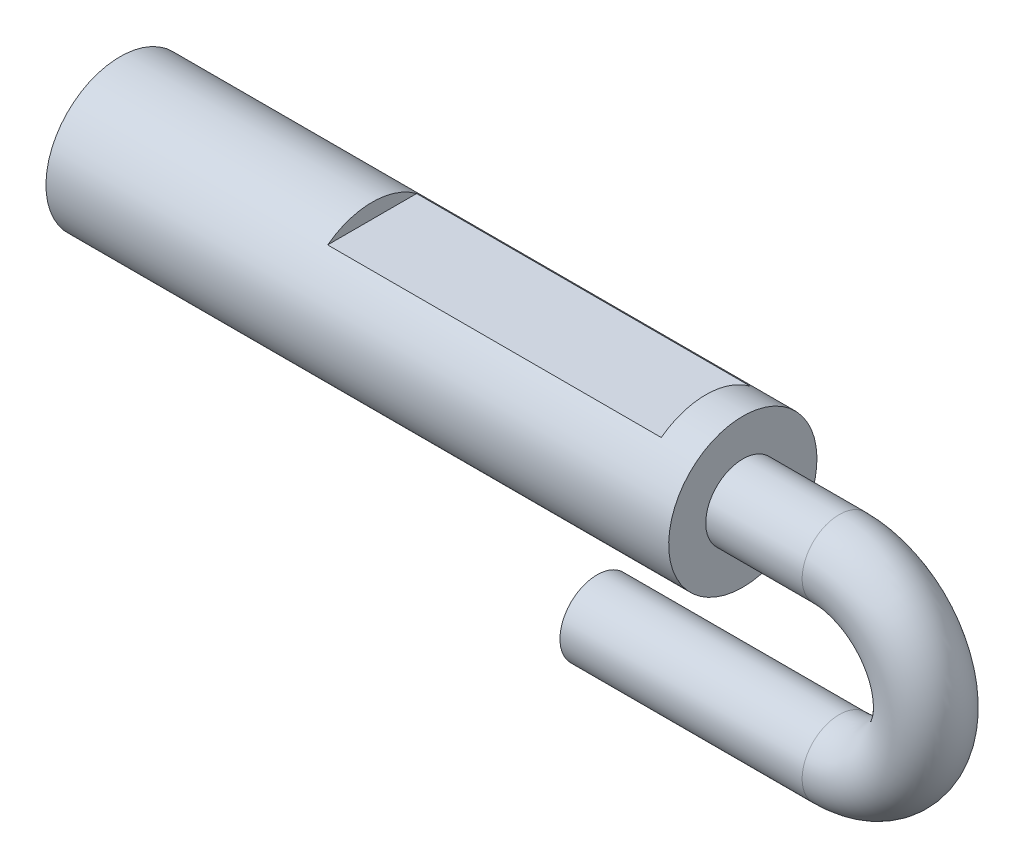
SolidWorks part; units mm, degrees
material "45"
ref_plane "前视基准面" through (0, 0, 0) normal (0, 0, 1) x (1, 0, 0)
ref_plane "上视基准面" through (0, 0, 0) normal (0, 1, 0) x (1, 0, 0)
ref_plane "右视基准面" through (0, 0, 0) normal (1, 0, 0) x (0, 0, -1)
sketch "草图1" plane through (0, 0, 0) normal (0, 0, 1) x (1, 0, 0)
  line L1 (-42, 0) -> (42, 0)
  line L2 (-42, 0) -> (-42, 10)
  line L3 (-42, 10) -> (42, 10)
  line L4 (42, 0) -> (42, 10)
  point P4 (0, 0)
  dimension "D1" = 10
  dimension "D2" = 84
revolve "旋转1" add sketch "草图1" angle 360 about L1
ref_plane "基准面1" through (0, 10, 0) normal (0, 1, 0) x (1, 0, 0)
sketch "草图2" plane through (0, 10, 0) normal (0, 1, 0) x (1, 0, 0)
  line L0 (42, -10) -> (42, 10) construction
  line L1 (-8, 17.2018) -> (37, 17.2018)
  line L2 (-8, 17.2018) -> (-8, -23.2445)
  line L3 (-8, -23.2445) -> (37, -23.2445)
  line L4 (37, 17.2018) -> (37, -23.2445)
  dimension "D1" = 5
  dimension "D2" = 45
extrude "切除-拉伸1" cut sketch "草图2" against normal blind 2
sketch "草图3" plane through (0, 0, 0) normal (0, 0, 1) x (1, 0, 0)
  line L0 (42, 0) -> (55, 0)
  line L1 (42, -10) -> (42, 10) construction
  line L2 (55, -23.3668) -> (22.3343, -23.3668)
  arc A0 (55, 0) -> (55, -23.3668) centre (55, -11.6834) cw
sweep "扫描1" add path "草图3" circular profile diameter 10 parameters "D3"=10
